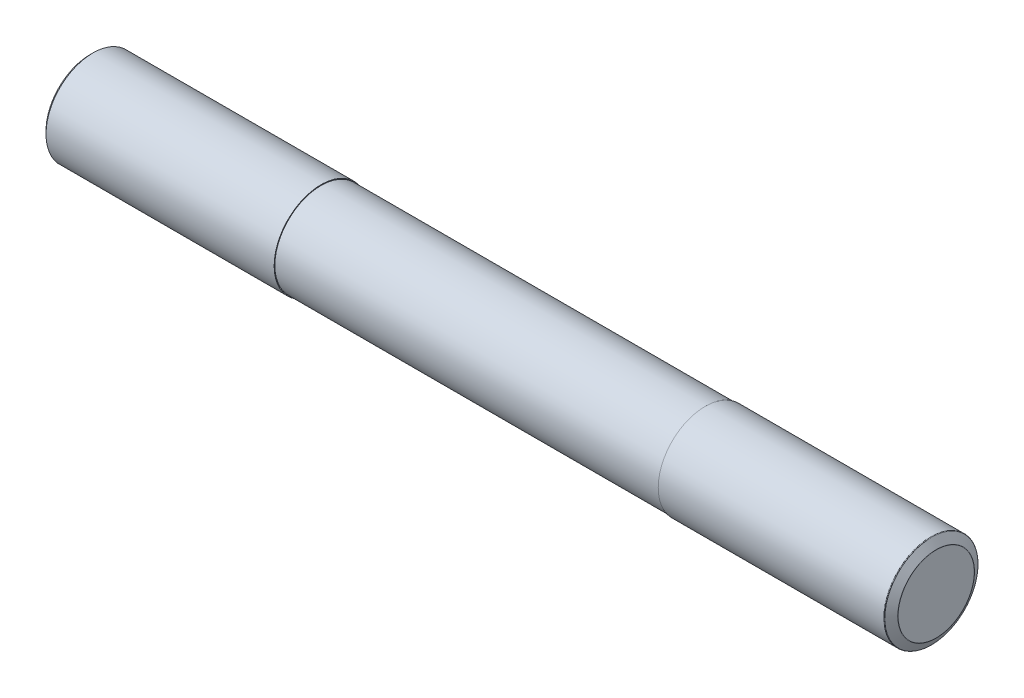
from build123d import *

# Parameters (mm, degrees)
CHAMFER_1_SIZE   = 2
CHAMFER_2_SIZE   = 6
CHAMFER_2_SIZE2  = 3.464101615
FILLET_1_R       = 0.5
MM_2_D           = 12
MM_2_DEPTH       = 10
MM_2_CSINK_D     = 18
MM_2_CSINK_ANGLE = 120
MM_2_TIP         = 3.605163714


with BuildPart() as part:
    # 草图1 → 旋转1 (revolve)
    with BuildSketch(Plane.XY, mode=Mode.PRIVATE) as revolve_1_sk:
        Polygon((0, 32.5), (160, 32.5), (160, 32), (426, 32), (426, 32.5), (586, 32.5), (586, 0), (0, 0), align=None)
    revolve(revolve_1_sk.sketch.rotate(Axis((-129.315789474, 0, 0), (1, 0, 0)), 90), axis=Axis((-129.315789474, 0, 0), (1, 0, 0)))

    # 倒角1
    chamfer_1_edges = [part.edges().sort_by_distance(p)[0] for p in [
        (0, 0, -32.5),
    ]]
    chamfer(chamfer_1_edges, length=CHAMFER_1_SIZE)

    # 倒角2
    chamfer_2_edges = [part.edges().sort_by_distance(p)[0] for p in [
        (586, 0, -32.5),
    ]]
    chamfer_2_side = [part.faces().sort_by_distance(p)[0] for p in [
        (586, 0, 0),
    ]]
    chamfer(chamfer_2_edges, length=CHAMFER_2_SIZE, length2=CHAMFER_2_SIZE2, reference=chamfer_2_side[0])

    # 圆角1
    fillet_1_edges = [part.edges().sort_by_distance(p)[0] for p in [
        (582.535898385, 0, -32.5),
        (586, 0, -26.5),
    ]]
    fillet(fillet_1_edges, radius=FILLET_1_R)

    # 大小mm 暗销孔2
    with Locations(Plane.XZ.offset(32.5)):
        with Locations((77, 0)):
            CounterSinkHole(MM_2_D / 2, MM_2_CSINK_D / 2, depth=MM_2_DEPTH, counter_sink_angle=MM_2_CSINK_ANGLE)
            with Locations((0, 0, -(MM_2_DEPTH + MM_2_TIP / 2))):  # 118° drill point
                Cone(0, MM_2_D / 2, MM_2_TIP, mode=Mode.SUBTRACT)


solid = part.part
